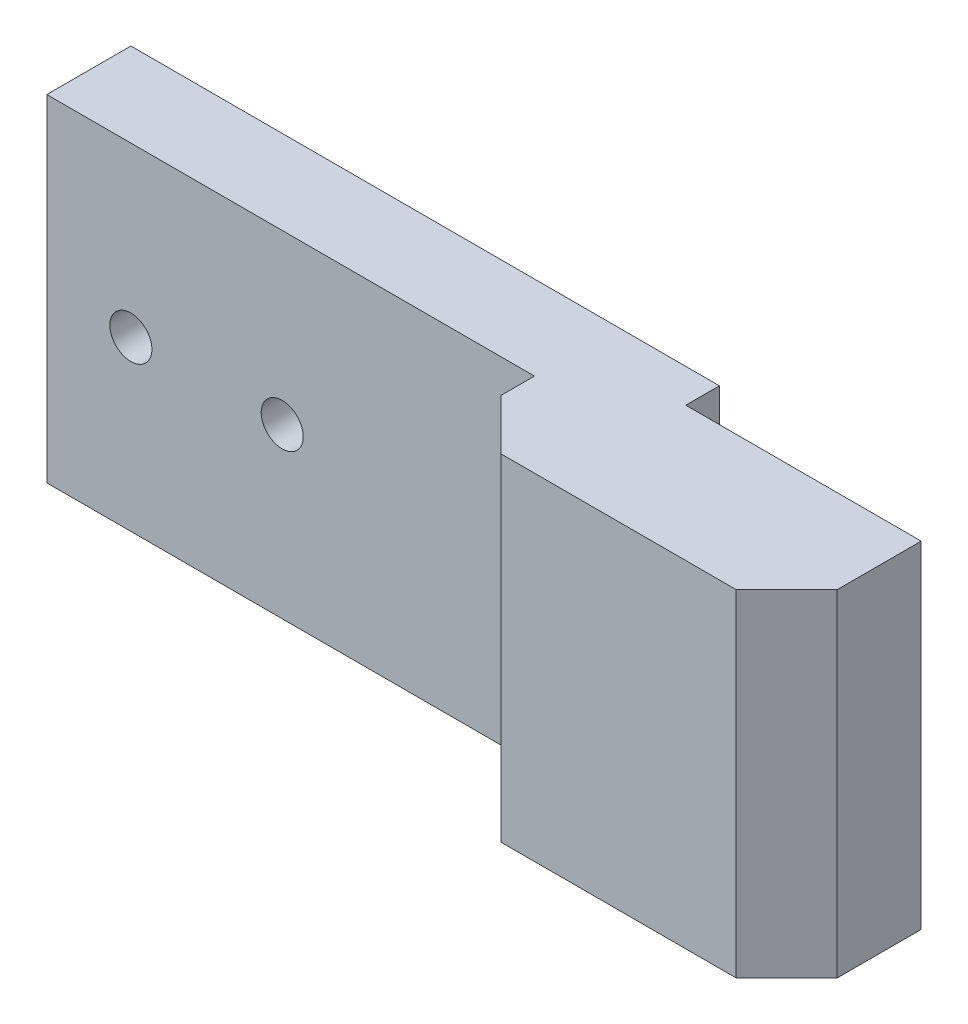
SolidWorks part; units mm, degrees
ref_plane "前视基准面" through (0, 0, 0) normal (0, 0, 1) x (1, 0, 0)
ref_plane "上视基准面" through (0, 0, 0) normal (0, 1, 0) x (1, 0, 0)
ref_plane "右视基准面" through (0, 0, 0) normal (1, 0, 0) x (0, 0, -1)
sketch "草图1" plane through (0, 0, 0) normal (0, 0, 1) x (1, 0, 0)
  line L1 (-15, 10) -> (15, 10)
  line L2 (-15, 10) -> (-15, -10)
  line L3 (-15, -10) -> (15, -10)
  line L4 (15, 10) -> (15, -10)
  line L5 (-15, 10) -> (15, -10) construction
  line L6 (-15, -10) -> (15, 10) construction
  point P0 (0, 0)
  dimension "1" = 30
  dimension "20" = 20
extrude "凸台-拉伸1" add sketch "草图1" along normal blind 5
sketch "草图2" plane through (15, 0, 0) normal (1, 0, 0) x (0, 0, -1)
  line L1 (0, 10) -> (-5, 10)
  line L2 (0, 10) -> (0, -10)
  line L3 (0, -10) -> (-5, -10)
  line L4 (-5, 10) -> (-5, -10)
  dimension "D1" = 20
  dimension "D2" = 5
extrude "凸台-拉伸2" add sketch "草图2" along normal blind 5
sketch "草图4" plane through (0, 0, 0) normal (0, 0, -1) x (-1, 0, 0)
  line L0 (-15.1639, 0) -> (10.8017, 0) construction
  line L1 (15, 0) -> (0, 0) construction
  line L2 (15, 10) -> (15, -10) construction
  line L3 (15, -5) -> (-20, -5)
  line L4 (15, -5) -> (15, 5)
  line L5 (15, 5) -> (-20, 5)
  line L6 (-20, -5) -> (-20, 5)
  line L7 (-20, -10) -> (-20, 10) construction
  dimension "D1" = 10
extrude "切除-拉伸1" cut sketch "草图4" against normal blind 1
sketch "草图5" plane through (0, 0, 5) normal (0, 0, 1) x (1, 0, 0)
  line L0 (20, 10) -> (-15, 10) construction
  line L1 (14, 10) -> (34, 10)
  line L2 (14, 10) -> (14, -10)
  line L3 (14, -10) -> (34, -10)
  line L4 (34, 10) -> (34, -10)
  line L6 (-15, 10) -> (-15, -10) construction
  dimension "D1" = 29
  dimension "D2" = 20
  dimension "D3" = 20
extrude "凸台-拉伸4" add sketch "草图5" along normal blind 5
sketch "草图6" plane through (34, 0, 0) normal (1, 0, 0) x (0, 0, -1)
  line L0 (3.0399, 0) -> (-13.7004, 0) construction
  line L2 (-8.4654, 0) -> (-5, 10)
  line L8 (-8.4654, 0) -> (-5, -10)
  line L9 (-10, -10) -> (-5, -10) construction
  line L11 (-5, -10) -> (-5, 10)
extrude "切除-拉伸2" [suppressed] cut sketch "草图6" against normal up to surface (14 mm away)
chamfer "倒角1" distance 3 angle 45 1 edges at (14, 0, 10)
chamfer "倒角2" distance 3 angle 45 1 edges at (34, 0, 10)
hole_wizard "M3x0.5 螺纹孔1" positions "草图13" profile "草图12" tap size "M3x0.5" standard "ANSI Metric" end condition through all
sketch "草图13" plane through (0, 0, 5) normal (0, 0, 1) x (1, 0, 0)
  line L0 (-1, 0) -> (-10, 0) construction
  line L1 (-10, 0) -> (-15, 0) construction
  line L2 (-15, 10) -> (-15, -10) construction
  point P0 (-10, 0)
  point P3 (-1, 0)
  dimension "D1" = 9
  dimension "D2" = 5
sketch "草图12" plane through (-10, 0, 5) normal (1, 0, 0) x (0, -1, 0)
  line L0 (0, 0) -> (0, 5)
  line L1 (0, 5) -> (1.25, 5)
  line L2 (1.25, 5) -> (1.25, 0)
  line L5 (1.25, 0) -> (0, 0)
  line L11 (0, -6.35) -> (0, 107.95) construction
  dimension "通孔螺纹孔钻头直径" = 2.5
  dimension "通孔螺纹孔钻头深度" = 5
cosmetic thread "孔螺蚊线1" parameters "D2"=3
cosmetic thread "孔螺蚊线2" parameters "D2"=3
other "移动面1" face at (27, 2.5, 5) parameters "D1"=3
